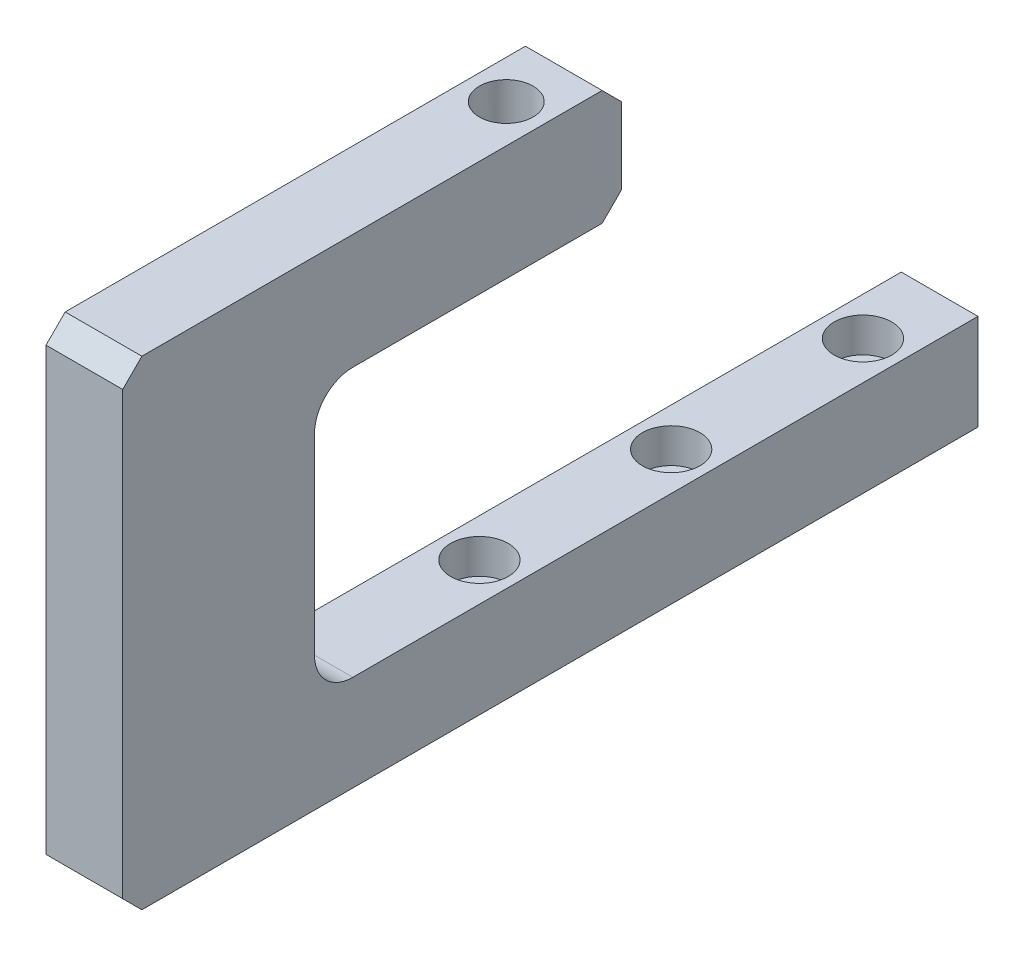
SolidWorks part; units mm, degrees
ref_plane "前视基准面" through (0, 0, 0) normal (0, 0, 1) x (1, 0, 0)
ref_plane "上视基准面" through (0, 0, 0) normal (0, 1, 0) x (1, 0, 0)
ref_plane "右视基准面" through (0, 0, 0) normal (1, 0, 0) x (0, 0, -1)
sketch "草图1" plane through (0, 0, 0) normal (0, 0, 1) x (1, 0, 0)
  line L1 (-10, 12.5) -> (10, 12.5)
  line L2 (-10, 12.5) -> (-10, -12.5)
  line L3 (-10, -12.5) -> (10, -12.5)
  line L4 (10, 12.5) -> (10, -12.5)
  line L5 (-10, 12.5) -> (10, -12.5) construction
  line L6 (-10, -12.5) -> (10, 12.5) construction
  point P0 (0, 0)
  dimension "D1" = 20
  dimension "D2" = 25
extrude "凸台-拉伸1" add sketch "草图1" along normal blind 223
hole_wizard "打孔尺寸(%根据)内六角圆柱头螺钉的类型1" positions "草图4" profile "草图5" counterbore size "M8" standard "GB" end condition through all
sketch "草图4" plane through (0, 12.5, 0) normal (0, 1, 0) x (1, 0, 0)
  line L0 (10, 0) -> (-10, 0) construction
  point P0 (0, -20)
  dimension "D1" = 20
sketch "草图5" plane through (0, 12.5, 20) normal (1, 0, 0) x (0, 0, 1)
  line L0 (0, 0) -> (0, 25)
  line L1 (0, 25) -> (4.5, 25)
  line L3 (4.5, 25) -> (4.5, 9)
  line L4 (4.5, 9) -> (7.5, 9)
  line L5 (7.5, 9) -> (7.5, 0)
  line L7 (7.5, 0) -> (0, 0)
  line L11 (0, -6.35) -> (0, 107.95) construction
  dimension "通孔孔直径" = 9
  dimension "通孔孔深度" = 25
  dimension "柱形沉头孔直径" = 15
  dimension "柱形沉头孔深度" = 9
pattern_linear "阵列(线性)1" count 3 spacing 50 along (0, 0, 1) of "打孔尺寸(%根据)内六角圆柱头螺钉的类型1"
sketch "草图6" plane through (0, 12.5, 0) normal (0, 1, 0) x (1, 0, 0)
  line L0 (10, -223) -> (10, 0) construction
  line L1 (-10, -223) -> (10, -223)
  line L2 (-10, -223) -> (-10, -173)
  line L3 (-10, -173) -> (10, -173)
  line L4 (10, -223) -> (10, -173)
  dimension "D1" = 50
extrude "凸台-拉伸3" add sketch "草图6" along normal blind 70
sketch "草图7" plane through (0, 82.5, 0) normal (0, 1, 0) x (1, 0, 0)
  line L0 (10, -173) -> (10, 0) construction
  line L1 (-10, -223) -> (10, -223)
  line L2 (-10, -223) -> (-10, -93)
  line L3 (-10, -93) -> (10, -93)
  line L4 (10, -223) -> (10, -93)
  dimension "D1" = 130
extrude "凸台-拉伸4" add sketch "草图7" along normal blind 30
hole_wizard "M16 螺纹孔1" positions "草图8" profile "草图9" tap size "M16" standard "GB"
sketch "草图8" plane through (0, 112.5, 0) normal (0, 1, 0) x (1, 0, 0)
  line L0 (0, -223) -> (0, -193.5708) construction
  line L1 (-10, -223) -> (10, -223) construction
  line L3 (10, -93) -> (-10, -93) construction
  point P0 (0, -113)
  dimension "D1" = 20
sketch "草图9" plane through (0, 112.5, 113) normal (1, 0, 0) x (0, 0, 1)
  line L0 (0, 0) -> (0, 42.206)
  line L1 (0, 42.206) -> (7, 38)
  line L2 (7, 38) -> (7, 0)
  line L5 (7, 0) -> (0, 0)
  line L10 (0, 42.206) -> (-7, 38) construction
  line L11 (0, -6.35) -> (0, 107.95) construction
  dimension "螺纹孔钻头直径" = 14
  dimension "螺纹孔钻头深度" = 38
  dimension "导头角度" = 118
cosmetic thread "孔螺蚊线1" parameters "D1"=30, "D2"=16
chamfer "倒角1" distance 5 angle 45 2 edges at (0, 112.5, 93) (0, 82.5, 93)
fillet "圆角1" radius 10 2 edges at (0, 82.5, 173) (0, 12.5, 173)
chamfer "倒角2" distance 5 angle 45 2 edges at (0, -12.5, 223) (0, 112.5, 223)
